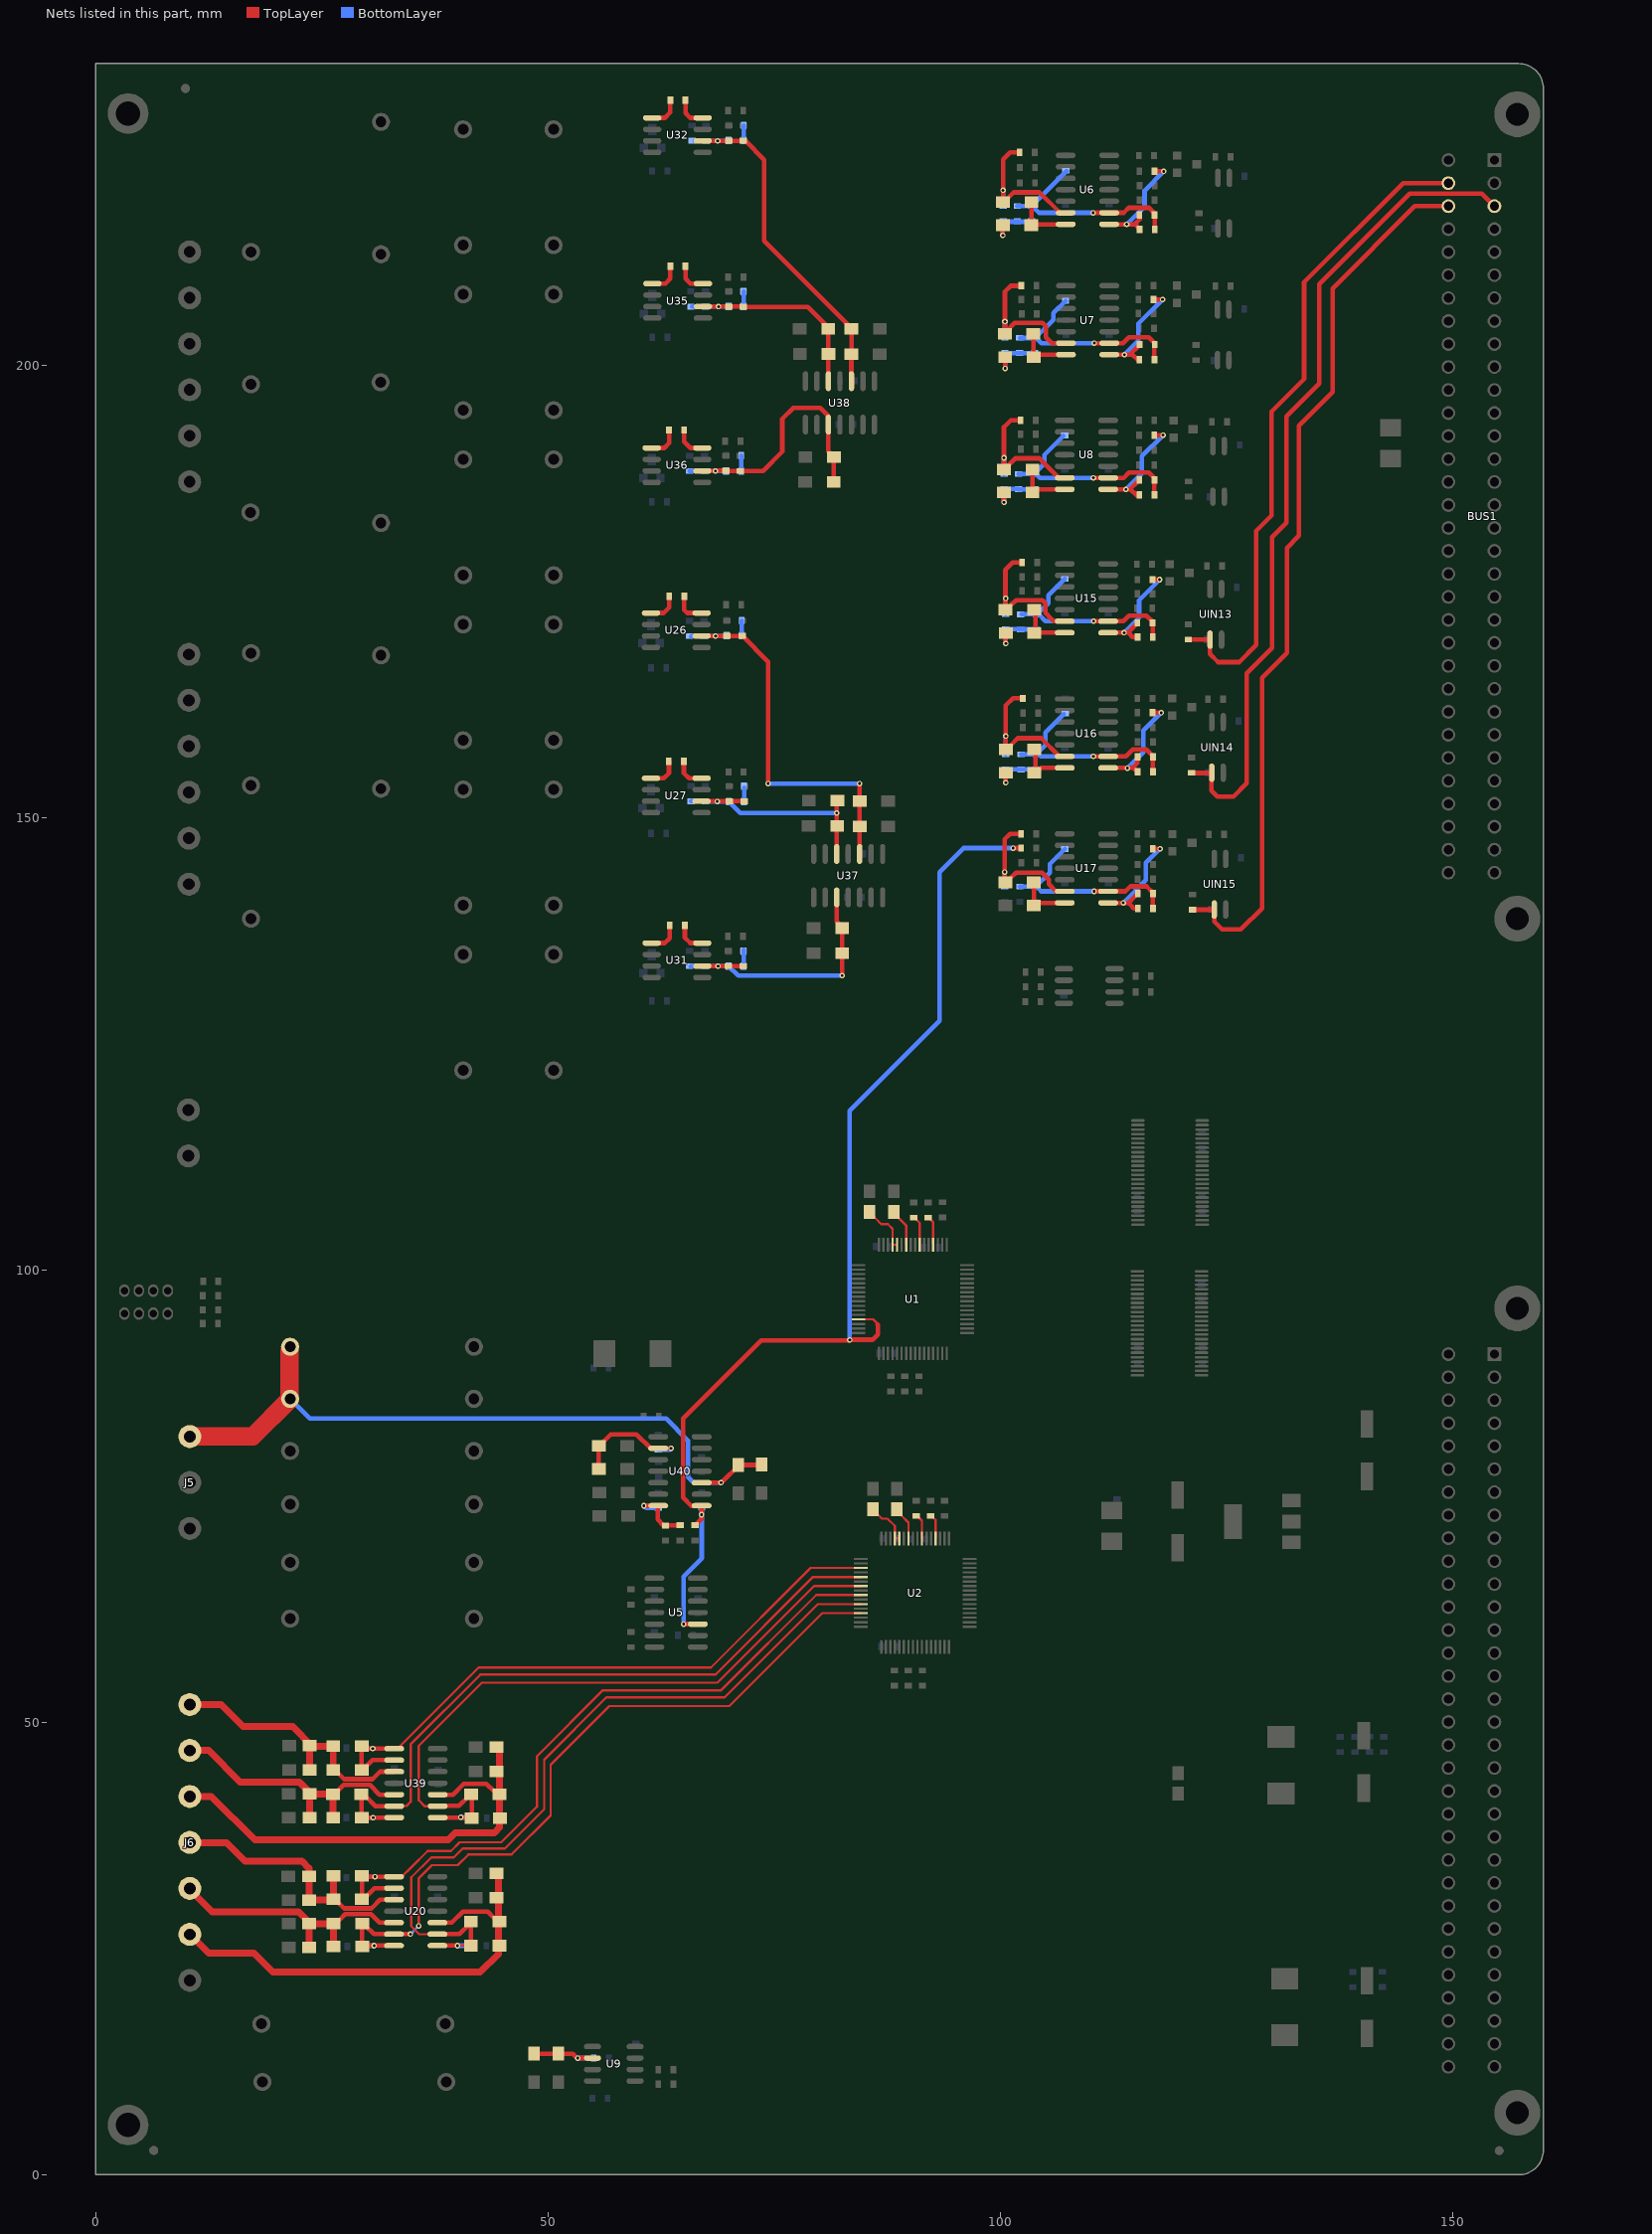
[diagram p0: the nets of this part, all layers, seen from the top]
# Altium PCB MISC80584.PCBDoc (part 5 of 7)
Units mm, origin at the board's own origin, x right, y up, seen from the top; angles counter-clockwise.
Board outline 160.02 x 233.3 mm, 4 copper layers (TopLayer, GND, POWER, BottomLayer); 386 components, 266 nets, 1374 pads, 640 vias.

## Via types
v1: diameter 0.61, hole 0.305, TopLayer to BottomLayer, 342 vias
v2: diameter 0.762, hole 0.381, TopLayer to BottomLayer, 197 vias
v3: diameter 0.508, hole 0.254, TopLayer to BottomLayer, 101 vias

## Nets (pads, with @x,y where several pads share a name; then routed paths per layer and width w, separated by ;. In a path a pad name is that pad's centre, name@x,y a point inside that pad or via, vN(x,y) a via of type N, cw(c..) or ccw(c..) an arc to the next point about the centre after c; other vN are vias at no path point) (continued)
ICC: C14.2 R85.1 R351.2 U1.61 U5.10 U40.8 | length 123.3
  TopLayer w0.254: U1.61@84.339,94.555 85.963,94.555 86.512,94.005
  TopLayer w0.508: v1(64.999,60.884) U5.10@66.56,60.884 ; C14.2@66.243,71.806 67.005,72.568 ; v1@67.005,72.974 67.005,73.939 66.98,73.965 65.837,73.965 64.948,74.854 64.948,83.617 73.558,92.227 83.261,92.227 83.337,92.304 85.877,92.304 86.462,92.888 86.462,93.548 86.462,93.955 86.436,93.98 ; v1(101.422,146.634) R351.2@102.286,146.634
  BottomLayer w0.254: R85.1@66.954,73.685 R85.1@66.98,73.66
  BottomLayer w0.508: v1(64.999,60.884) 64.999,66.142 67.005,68.148 R85.1@67.005,73.787 ; v1(83.363,92.278) 83.363,117.627 93.269,127.533 93.269,143.967 95.936,146.634 v1(101.422,146.634)
  other v1: 66.98,72.974
ICCIN: D95.K D97.A J5.1 R8.2 R9.2 U40.10 | length 78.5
  TopLayer w0.508: U40.10@66.992,76.505 v1(69.139,76.505) 69.164,76.505 71.12,78.461 D97.A@73.457,78.461
  TopLayer w2.032: J5.1@10.414,81.61 17.348,81.61 21.438,85.7 R9.2@21.438,91.034
  BottomLayer w0.508: R8.2@21.971,85.319 23.698,83.591 63.068,83.591 65.507,81.153 65.507,77.114 66.116,76.505 v1(69.139,76.505)
IILA: D28.K D33.A J6.1 R23.1 R24.1 U39.3 | length 29.4
  TopLayer w0.508: D33.A@26.67,44.577 27.495,43.752 30.594,43.752 31.42,44.577 U39.3@33.008,44.577
  TopLayer w0.762: J6.1@10.414,51.994 13.894,51.994 16.307,49.581 21.768,49.581 23.952,47.396 D28.K@26.264,47.396 D33.A@26.264,45.187 ; R24.1@23.622,47.117 23.673,47.066 R23.1@23.673,44.755
IILB: D26.K D31.A J6.2 R27.1 R29.1 U39.5 | length 29.5
  TopLayer w0.508: D31.A@26.746,42.443 27.407,43.104 30.328,43.104 31.394,42.037 U39.5@33.008,42.037
  TopLayer w0.762: J6.2@10.414,46.914 12.497,46.914 15.977,43.434 22.53,43.434 23.851,42.113 D31.A@26.162,42.113 ; R29.1@23.647,39.649 R27.1@23.647,42.113 ; D26.K@26.238,39.726 D31.A@26.238,42.062
IILC: D27.K D32.A J6.3 R32.1 R35.1 U39.10 | length 52.6
  TopLayer w0.508: U39.10@37.808,42.037 39.497,42.037 40.691,43.231 43.205,43.231 D32.A@44.044,42.393
  TopLayer w0.762: J6.3@10.414,41.834 12.802,41.834 17.602,37.033 38.989,37.033 39.776,37.821 44.069,37.821 44.653,38.405 R32.1@44.653,47.168
IISA: D62.K D65.A J6.4 R25.1 R26.1 U20.3 | length 29
  TopLayer w0.508: D65.A@26.721,30.226 27.483,29.464 30.485,29.464 30.582,29.56 30.582,29.566 31.445,30.429 U20.3@32.982,30.429
  TopLayer w0.762: J6.4@11.379,36.728 14.503,36.728 16.535,34.696 22.809,34.696 23.571,33.934 ; R26.1@23.597,32.868 23.597,33.934 ; R26.1@23.622,32.918 R25.1@23.622,30.378 26.162,30.378 26.314,30.531 D62.K@26.314,32.868
IISB: D63.K D80.A J6.5 R30.1 R31.1 U20.5 | length 28.8
  TopLayer w0.508: D63.K@26.949,28.194 27.572,28.816 30.442,28.816 31.369,27.889 U20.5@32.982,27.889
  TopLayer w0.762: J6.5@10.414,31.674 10.414,31.547 12.878,29.083 22.454,29.083 R31.1@23.749,27.788 ; R30.1@23.622,25.324 23.622,27.661 R31.1@23.749,27.788 ; R31.1@23.774,27.813 R31.1@23.749,27.788 ; D80.A@26.314,25.806 26.314,27.737 26.289,27.762 23.774,27.762 R31.1@23.749,27.788
IISC: D64.K D81.A J6.6 R36.1 R38.1 U20.10 | length 52.4
  TopLayer w0.508: U20.10@37.782,27.889 39.37,27.889 40.589,29.108 43.332,29.108 D81.A@44.018,28.423
  TopLayer w0.762: J6.6@10.414,26.594 12.497,24.511 17.526,24.511 19.609,22.428 42.52,22.428 44.526,24.435 R38.1@44.526,33.122
ILA: C12.2 D28.A D33.K U2.51 U39.1 U39.2 | length 70.3
  TopLayer w0.254: U39.1@33.376,47.117 42.342,56.083 68.021,56.083 79.032,67.094 U2.51@84.593,67.094
  TopLayer w0.508: D33.K@29.413,44.679 D33.K@29.413,44.78 29.413,47.117 30.607,47.117 v1(30.632,47.117) U39.1@33.008,47.117 U39.1@33.376,47.117 ; D33.K@29.947,45.187 30.607,45.847 U39.2@33.008,45.847
  BottomLayer w0.508: C12.2@29.54,47.117 v1(30.632,47.117)
ILB: C20.2 D26.A D31.K U2.53 U39.6 U39.7 | length 75.7
  TopLayer w0.254: U39.6@33.376,40.792 34.366,40.792 34.823,41.25 34.823,47.6 42.52,55.296 68.504,55.296 79.302,66.094 U2.53@84.593,66.094
  TopLayer w0.508: D26.A@29.312,39.929 29.388,40.005 D31.K@29.388,42.062 ; D31.K@29.82,41.885 30.937,40.767 U39.6@33.008,40.767 ; D26.A@29.87,39.522 29.896,39.497 U39.7@33.008,39.497
  BottomLayer w0.508: C20.2@29.413,39.497 v1(30.683,39.497)
ILC: C23.2 D27.A D32.K U2.55 U39.8 U39.9 | length 74.6
  TopLayer w0.254: U39.9@37.186,40.742 36.398,40.742 35.712,41.427 35.712,47.422 42.697,54.407 68.732,54.407 79.419,65.094 U2.55@84.593,65.094
  TopLayer w0.508: U39.8@37.808,39.497 v1@40.361,39.497 ; U39.9@38.43,40.792 40.183,40.792 41.123,41.732 41.529,41.732 41.58,41.681 41.58,39.522 41.554,39.497 v1@40.361,39.497 ; v1(40.361,39.548) v1@40.361,39.497
  BottomLayer w0.508: v1(40.361,39.548) 40.386,39.522 C23.2@41.478,39.522
IPR1: BUS1.C2 R600.2 UIN13.3 | length 72.8
  TopLayer w0.508: R600.2@120.777,169.672 123.139,169.672 UIN13.3@123.165,169.647 ; UIN13.3@123.165,169.443 123.165,168.097 124.079,167.183 126.39,167.183 128.27,169.062 128.27,181.686 129.972,183.388 129.972,194.869 133.579,198.476 133.579,209.169 144.526,220.116 BUS1.C2@149.53,220.116
IPR2: BUS1.A3 R601.2 UIN14.3 | length 91.6
  TopLayer w0.508: R601.2@121.209,154.94 123.241,154.94 123.342,155.042 123.342,152.984 124.003,152.324 125.781,152.324 127.254,153.797 127.254,165.938 130.048,168.732 130.048,181 131.623,182.575 131.623,194.361 135.255,197.993 135.255,208.966 145.237,218.948 153.238,218.948 BUS1.A3@154.61,217.576
IPR3: BUS1.C3 R602.2 UIN15.3 | length 98.6
  TopLayer w0.508: R602.2@121.437,139.827 123.622,139.827 123.673,139.878 123.647,139.878 UIN15.3@123.647,139.852 123.647,138.506 124.511,137.643 126.594,137.643 128.93,139.979 128.93,165.456 131.674,168.199 131.674,179.807 133.02,181.153 133.02,193.319 136.728,197.028 136.728,208.483 145.821,217.576 BUS1.C3@149.53,217.576
ISA: C13.2 D62.A D65.K U2.57 U20.1 U20.2 | length 78.8
  TopLayer w0.254: U20.1@32.982,32.969 33.858,32.969 34.874,33.985 ; 35.001,34.112 34.874,33.985 ; U2.57@84.593,64.094 79.664,64.094 69.139,53.569 56.083,53.569 48.793,46.279 48.793,40.716 44.844,36.767 40.246,36.767 39.294,35.814 36.703,35.814 34.874,33.985
  TopLayer w0.508: D65.K@29.439,30.505 D62.A@29.439,32.893 ; D62.A@29.489,32.969 v1(30.886,32.969) U20.1@32.982,32.969 ; D65.K@29.947,30.81 30.836,31.699 U20.2@32.982,31.699
  BottomLayer w0.508: C13.2@29.388,32.868 29.464,32.944 v1@30.886,32.944
ISB: C21.2 D63.A D80.K U2.61 U20.6 U20.7 | length 87.1
  TopLayer w0.254: D80.K@29.693,25.349 32.969,25.349 U20.7@32.982,25.349 ; U20.6@32.969,26.492 U20.6@33.02,26.543 ; v1(35.712,27.534) 35.712,32.791 35.916,32.995 ; 35.738,32.817 35.916,32.995 ; U2.61@84.593,62.094 80.331,62.094 70.053,51.816 56.769,51.816 50.292,45.339 50.292,39.751 45.974,35.433 41.224,35.433 40.03,34.239 37.16,34.239 35.916,32.995
  TopLayer w0.508: U20.7@33.147,25.349 33.122,25.375 29.642,25.375 29.464,25.552 29.464,27.254 29.794,27.584 30.759,26.619 U20.6@32.982,26.619 v1@34.773,26.619
  BottomLayer w0.254: v1(34.798,26.619) v1(35.712,27.534)
  BottomLayer w0.508: C21.2@29.515,25.273 29.591,25.349 v1(30.785,25.349)
ISC: C27.2 D64.A D81.K U2.59 U20.8 U20.9 | length 87
  TopLayer w0.254: U20.9@37.541,26.619 35.763,26.619 34.9,27.483 34.9,32.893 37.109,35.103 39.599,35.103 40.589,36.093 45.237,36.093 49.581,40.437 49.581,45.898 56.464,52.781 69.52,52.781 79.832,63.094 U2.59@84.593,63.094 ; U20.8@37.782,25.349 37.795,25.362 U20.8@37.795,25.375 ; U20.8@38.456,25.375 v1@40.005,25.375 ; v1(40.005,25.349) v1@40.005,25.375 ; D64.A@41.478,25.375 41.199,25.375 v1@40.005,25.375
  TopLayer w0.508: U20.9@37.782,26.619 40.234,26.619 D81.K@41.326,27.711 ; U20.8@38.049,25.375 v1@40.005,25.375 ; D64.A@41.199,25.375 41.478,25.654 D81.K@41.478,27.991
  BottomLayer w0.508: v1(40.005,25.349) 41.377,25.349 C27.2@41.402,25.375
IU1: C104.1 C113.1 C139.2 D10.K D14.A R119.1 R120.1 U32.6 U38.3 | length 39.9
  TopLayer w0.508: U32.6@67.107,224.79 v1(68.758,224.79) C139.2@71.679,224.79 ; C139.2@71.577,224.815 C139.2@71.857,224.815 ; C139.2@71.857,224.765 73.914,222.707 73.914,213.741 83.566,204.089 83.566,201.32 D10.K@83.541,201.295 ; U38.3@83.541,198.234 D10.K@83.541,201.244
  BottomLayer w0.508: R120.1@66.192,224.79 R119.1@67.488,224.79 v1(68.758,224.79) 69.901,224.79 C113.1@69.926,224.815
IU2: C126.2 C142.1 C143.1 D24.K D29.A R110.1 R111.1 U35.6 U38.5 | length 24.7
  TopLayer w0.508: U35.6@67.132,206.477 C142.1@69.977,206.477 71.577,206.477 71.603,206.451 78.74,206.451 81.001,204.191 D29.A@81.001,201.244 U38.5@81.001,198.234
  BottomLayer w0.508: R111.1@65.913,206.477 R110.1@67.412,206.477 v1@68.885,206.477 ; v1(68.859,206.477) v1@68.885,206.477 ; C143.1@69.774,206.477 v1@68.885,206.477
IU3: C130.1 C132.1 C136.2 D25.K D30.A R105.1 R106.1 U36.6 U38.10 | length 29.3
  TopLayer w0.508: U36.6@67.589,188.316 v1(68.504,188.316) ; v1@68.631,188.316 68.656,188.341 C130.1@69.672,188.341 ; C130.1@69.901,188.316 C136.2@71.272,188.316 73.762,188.316 75.895,190.449 75.895,194.056 77.114,195.275 80.112,195.275 80.975,194.412 U38.10@80.975,194.005 ; U38.10@81.001,193.434 81.001,190.5 D25.K@81.585,189.916 ; D30.A@81.509,187.274 81.585,187.35 D25.K@81.585,189.916 ; D25.K@81.585,190.094 D25.K@81.585,189.916 ; D25.K@81.661,189.84 D25.K@81.585,189.916
  BottomLayer w0.508: R105.1@65.659,188.316 67.158,188.316 R106.1@67.208,188.265 ; R106.1@67.488,188.341 67.513,188.316 v1(68.504,188.316) C132.1@69.698,188.316
IUA: C82.1 C83.1 C85.2 D8.K D12.A R138.1 R139.1 U26.6 U37.3 | length 43.3
  TopLayer w0.508: U26.6@66.98,170.078 v1(68.529,170.078) C85.2@71.399,170.078 ; C85.2@71.476,170.104 74.346,167.234 v1(74.346,153.772) ; v1(84.43,153.772) 84.43,152.298 D12.A@84.531,152.197 ; U37.3@84.455,145.986 D8.K@84.455,149.047 84.455,151.663 D12.A@84.506,151.714
  BottomLayer w0.508: R138.1@65.837,170.028 65.862,170.053 68.504,170.053 v1(68.529,170.078) C83.1@69.748,170.078 ; v1(74.346,153.772) v1(84.43,153.772)
IUB: C88.1 C89.1 C93.2 D11.K D15.A R131.1 R133.1 U27.6 U37.5 | length 27.3
  TopLayer w0.508: U27.6@66.98,151.816 v1@68.732,151.816 ; v1(68.707,151.79) v1@68.732,151.816 ; C93.2@71.73,151.765 71.679,151.816 71.018,151.816 v1@68.732,151.816 ; D11.K@81.89,151.943 81.915,151.917 81.915,151.867 U37.5@81.915,145.986
  BottomLayer w0.508: R131.1@65.837,151.816 67.31,151.816 67.361,151.765 C89.1@69.926,151.765 ; C89.1@70.002,151.79 71.272,150.52 v1(81.915,150.52)
IUC: C96.1 C97.1 C101.2 D9.K D13.A R125.1 R126.1 U31.6 U37.10 | length 29.4
  TopLayer w0.508: U31.6@67.564,133.604 v1(68.809,133.604) ; v1@68.91,133.604 69.901,133.604 C96.1@69.952,133.553 ; C96.1@70.079,133.604 71.145,133.604 C101.2@71.577,133.604 ; U37.10@81.915,141.186 81.915,138.532 82.525,137.922 D9.K@82.525,137.795 D13.A@82.525,135.382 ; D13.A@82.474,134.976 82.525,134.925 v1(82.525,132.537)
  BottomLayer w0.508: R126.1@65.761,133.553 65.811,133.604 R125.1@67.335,133.604 v1(68.809,133.604) C97.1@69.799,133.604 ; C97.1@69.952,133.604 71.018,132.537 v1(82.525,132.537)
NetC4_1: C4.1 R150.2 R450.1 U6.8 | length 13.6
  TopLayer w0.508: U6.8@112.026,215.57 v1(113.97,215.57) 114.884,215.57 114.91,215.544 ; 114.859,215.595 114.91,215.646 ; R450.1@115.392,216.687 115.392,216.129 114.91,215.646 ; C4.1@115.443,215.011 114.91,215.544 ; R150.2@117.043,221.412 v1(118.059,221.412) ; 114.91,215.544 114.91,215.646
  BottomLayer w0.508: v1(113.97,215.57) 115.951,217.551 115.951,219.304 v1(118.059,221.412)
NetC4_2: C4.2 R76.1 R100.1 R132.1 R450.2 U6.9 | length 22.7
  TopLayer w0.508: v1(110.261,216.84) U6.9@112.026,216.84 113.64,216.84 114.198,217.399 116.434,217.399 117.069,216.764 C4.2@117.069,215.316
  BottomLayer w0.508: R132.1@101.879,217.576 R100.1@103.429,217.576 ; R100.1@103.454,217.576 107.315,221.437 R76.1@107.366,221.437 ; R100.1@103.632,217.475 104.267,216.84 v1(110.261,216.84)
NetC5_1: C5.1 R151.2 R451.1 U7.8 | length 13.6
  TopLayer w0.508: U7.8@112.052,201.168 v1(113.716,201.168) 114.605,201.168 115.138,200.635 C5.1@115.443,200.635 ; 114.351,201.193 R451.1@115.24,202.082 ; R151.2@117.043,207.239 117.907,207.239 v1(117.932,207.264)
  BottomLayer w0.508: v1(113.716,201.168) 115.265,202.717 115.265,204.597 v1(117.932,207.264)
NetC5_2: C5.2 R86.1 R108.1 R146.1 R451.2 U7.9 | length 22.7
  TopLayer w0.508: v1(110.388,202.438) U7.9@112.052,202.438 113.563,202.438 114.211,203.086 116.395,203.086 117.018,202.463 C5.2@117.018,200.66
  BottomLayer w0.508: R146.1@102.21,202.997 103.861,202.997 105.867,205.003 105.867,205.765 R86.1@107.213,207.112 ; R108.1@104.013,202.971 104.546,202.438 v1(110.388,202.438)
NetC6_1: C6.1 R152.2 R452.1 U8.8 | length 13.5
  TopLayer w0.508: U8.8@111.925,186.284 114.3,186.284 R452.1@115.189,187.173 ; 114.402,186.284 115.037,185.649 C6.1@115.367,185.649 ; R152.2@117.018,192.278 v1(117.983,192.278)
  BottomLayer w0.508: v1(113.894,186.284) 115.646,188.036 115.646,189.941 v1(117.983,192.278)
NetC6_2: C6.2 R87.1 R117.1 R147.1 R452.2 U8.9 | length 22.6
  TopLayer w0.508: v1(110.287,187.554) U8.9@111.925,187.554 113.64,187.554 114.211,188.125 116.421,188.125 117.018,187.528 C6.2@117.018,185.877
  BottomLayer w0.508: R147.1@102.032,187.985 103.734,187.985 104.877,189.128 104.877,190.094 R87.1@106.959,192.176 ; R117.1@103.988,187.935 104.369,187.554 v1(110.287,187.554)
NetC11_2: C11.2 R5.2 R93.1 U40.7 | length 7.4
  TopLayer w0.508: v1(60.604,73.965) U40.7@62.192,73.965 ; U40.7@62.128,73.812 62.128,72.441 62.763,71.806 C11.2@64.618,71.806
  BottomLayer w0.508: v1@60.63,73.965 60.858,73.736 R93.1@62.179,73.736
NetC15_1: C15.1 R375.2 R459.1 U15.8 | length 12.8
  TopLayer w0.508: U15.8@111.925,170.434 114.097,170.434 C15.1@114.986,171.323 ; 114.249,170.332 114.605,169.977 R459.1@115.164,169.977 ; R375.2@116.815,176.301 v1(117.602,176.301)
  BottomLayer w0.508: v1(113.69,170.434) 115.341,172.085 115.341,174.041 v1(117.602,176.301)
NetC15_2: C15.2 R360.1 R364.1 R372.1 R459.2 U15.9 | length 21.6
  TopLayer w0.508: v1(110.312,171.704) U15.9@111.354,171.704 ; U15.9@111.925,171.704 113.589,171.704 114.224,172.339 116.154,172.339 116.84,171.653 R459.2@116.84,170.002
  BottomLayer w0.508: R364.1@102.362,172.466 R372.1@104.013,172.466 R372.1@104.064,172.466 ; R360.1@107.112,176.378 105.308,174.574 105.308,173.711 R372.1@104.064,172.466 ; v1(110.312,171.704) 105.004,171.704 104.242,172.466 R372.1@104.064,172.466
NetC16_1: C16.1 R376.2 R460.1 U16.8 | length 13
  TopLayer w0.508: U16.8@111.925,155.499 v1@114.021,155.499 ; v1(114.046,155.473) v1@114.021,155.499 ; 114.681,155.575 115.138,156.032 115.138,156.667 R460.1@115.189,156.718 ; C16.1@114.986,155.245 114.732,155.499 v1@114.021,155.499 ; R376.2@116.967,161.595 v1(117.78,161.595)
  BottomLayer w0.508: v1(114.046,155.473) 115.799,157.226 115.799,159.614 v1(117.78,161.595)
NetC16_2: C16.2 R361.1 R365.1 R373.1 R460.2 U16.9 | length 22.5
  TopLayer w0.508: v1(110.287,156.769) U16.9@111.925,156.769 113.894,156.769 114.656,157.531 116.154,157.531 116.764,156.921 116.764,156.87 116.84,156.794 C16.2@116.84,155.143
  BottomLayer w0.508: R365.1@102.311,156.997 103.988,156.997 R373.1@104.013,157.023 105.004,158.013 105.004,159.41 R361.1@107.036,161.442 ; R373.1@104.165,157.074 104.47,156.769 v1(110.287,156.769)
NetC17_1: C17.1 R377.2 R461.1 U17.8 | length 13
  TopLayer w0.508: U17.8@111.925,140.589 114.173,140.589 R461.1@115.011,141.427 ; 114.275,140.487 114.783,139.979 C17.1@115.214,139.979 ; R377.2@116.84,146.558 v1(117.653,146.558)
  BottomLayer w0.508: v1(113.589,140.589) 116.103,143.104 116.103,144.323 116.103,145.009 v1(117.653,146.558)
NetC17_2: C17.2 R362.1 R366.1 R374.1 R461.2 U17.9 | length 22.3
  TopLayer w0.508: v1(110.363,141.859) U17.9@111.925,141.859 113.843,141.859 114.389,142.405 116.167,142.405 116.84,141.732 C17.2@116.84,140.132
  BottomLayer w0.508: R374.1@102.159,142.392 R366.1@103.835,142.392 103.911,142.392 105.461,143.942 105.461,144.882 R362.1@107.112,146.533 ; R366.1@104.038,142.342 104.521,141.859 v1(110.363,141.859)
NetC19_2: C19.2 U1.39 | length 3
  TopLayer w0.254: C19.2@90.678,105.639 91.089,105.228 U1.39@91.089,102.805
NetC22_2: C22.2 U1.36 | length 3.1
  TopLayer w0.254: C22.2@92.151,105.715 92.589,105.277 U1.36@92.589,102.805
NetC25_2: C25.2 U2.39 | length 2.6
  TopLayer w0.254: C25.2@90.907,72.746 91.343,72.31 U2.39@91.343,70.344
NetC26_2: C26.2 U2.36 | length 2.4
  TopLayer w0.254: C26.2@92.583,72.644 92.837,72.39 92.837,71.869 92.835,71.866 92.835,70.352 U2.36@92.843,70.344
NetC83_2: C83.2 R137.1 | length 1.7
  BottomLayer w0.508: R137.1@71.425,171.78 71.425,170.688 71.425,170.129 C83.2@71.45,170.104
NetC84_1: C84.1 U26.8 | length 3.4
  TopLayer w0.508: C84.1@65.049,174.32 65.049,172.949 65.38,172.618 U26.8@66.98,172.618
NetC84_2: C84.2 U26.1 | length 3.4
  TopLayer w0.508: U26.1@61.392,172.618 62.789,172.618 63.398,173.228 C84.2@63.398,174.371
NetC89_2: C89.2 R130.1 | length 1.5
  BottomLayer w0.508: C89.2@71.679,151.79 71.679,152.298 R130.1@71.679,153.289
NetC92_1: C92.1 U27.8 | length 3.5
  TopLayer w0.508: C92.1@65.024,156.185 65.024,154.915 65.583,154.356 U27.8@66.98,154.356
NetC92_2: C92.2 U27.1 | length 3.5
  TopLayer w0.508: U27.1@61.392,154.356 62.814,154.356 63.373,154.915 C92.2@63.373,156.21
NetC97_2: C97.2 R124.1 | length 1.8
  BottomLayer w0.508: C97.2@71.628,133.604 71.628,134.264 R124.1@71.628,135.255 R124.1@71.628,135.382
NetC100_1: C100.1 U31.8 | length 3.6
  TopLayer w0.508: C100.1@65.126,138.125 C100.1@65.126,138.1 65.126,136.754 65.735,136.144 U31.8@67.056,136.144
NetC100_2: C100.2 U31.1 | length 3.5
  TopLayer w0.508: U31.1@61.468,136.144 62.916,136.144 63.449,136.677 C100.2@63.449,137.998
NetC113_2: C113.2 R118.1 | length 1.7
  BottomLayer w0.508: C113.2@71.628,224.765 71.653,224.79 C113.2@71.653,224.815 71.653,225.577 R118.1@71.653,226.492
NetC118_1: C118.1 U32.8 | length 3.4
  TopLayer w0.508: C118.1@65.227,229.184 65.227,227.838 65.735,227.33 U32.8@67.107,227.33
NetC118_2: C118.2 U32.1 | length 3.6
  TopLayer w0.508: U32.1@61.519,227.33 62.916,227.33 63.525,227.94 C118.2@63.525,229.286 C118.2@63.525,229.311
NetC121_2: C121.2 U1.44 U1.45 | length 4.8
  TopLayer w0.254: C121.2@86.081,105.842 86.843,105.08 87.579,105.08 88.101,104.558 88.101,102.805 U1.44@88.589,102.805
NetC122_2: C122.2 U1.42 | length 3.6
  TopLayer w0.254: C122.2@88.544,105.994 89.589,104.95 U1.42@89.589,102.805
NetC123_2: C123.2 U2.44 U2.45 | length 4.4
  TopLayer w0.254: C123.2@86.411,73.05 86.919,72.542 87.528,72.542 88.343,71.728 U2.45@88.343,70.357 ; U2.45@88.341,70.358 U2.45@88.343,70.357 ; U2.45@88.343,70.344 U2.45@88.343,70.357 ; U2.44@88.843,70.344 88.355,70.344 U2.45@88.343,70.357
NetC124_2: C124.2 U2.42 | length 3
  TopLayer w0.254: C124.2@89.002,72.949 89.843,72.108 U2.42@89.843,70.344
NetC125_1: C125.1 U35.8 | length 3.5
  TopLayer w0.508: C125.1@65.202,210.896 65.202,209.55 65.735,209.017 U35.8@67.132,209.017
NetC125_2: C125.2 U35.1 | length 3.5
  TopLayer w0.508: U35.1@61.544,209.017 62.992,209.017 63.525,209.55 C125.2@63.525,210.82
NetC132_2: C132.2 R414.1 | length 1.7
  BottomLayer w0.508: C132.2@71.374,188.29 C132.2@71.374,188.316 R414.1@71.374,189.992
NetC135_1: C135.1 U36.8 | length 3.6
  TopLayer w0.508: C135.1@65.049,192.837 65.049,191.567 65.761,190.856 U36.8@67.056,190.856
NetC135_2: C135.2 U36.1 | length 3.4
  TopLayer w0.508: U36.1@61.468,190.856 62.84,190.856 63.398,191.414 C135.2@63.398,192.684
NetC143_2: C143.2 R113.1 | length 1.7
  BottomLayer w0.508: C143.2@71.628,206.477 R113.1@71.628,208.153
NetD1_A: D1.A D2.K R11.2 U9.2 | length 8.1
  TopLayer w0.508: D2.K@48.768,13.386 52.73,13.386 53.188,12.929 U9.2@54.927,12.929
  BottomLayer w0.508: v1(53.289,12.929) R11.2@54.991,12.929
NetD16_A: D16.A D20.K U6.7 | length 5.5
  TopLayer w0.508: D16.A@103.454,218.034 103.454,215.697 103.581,215.57 U6.7@106.578,215.57
NetD16_K: D16.K R57.1 R67.2 U6.6 | length 15.8
  TopLayer w0.508: D16.K@100.305,218.415 100.305,222.733 101.092,223.52 R57.1@102.133,223.52 ; D16.K@100.813,218.44 101.473,219.1 104.343,219.1 106.604,216.84 U6.6@107.226,216.84
  BottomLayer w0.508: R67.2@100.305,217.576 v1(100.305,219.329)
NetD17_A: D17.A D21.K U7.7 | length 5.7
  TopLayer w0.508: D17.A@103.657,203.479 103.657,201.066 103.708,201.016 103.861,201.168 U7.7@106.883,201.168
NetD17_K: D17.K R58.1 R70.2 U7.6 | length 17.1
  TopLayer w0.508: D17.K@100.508,203.479 100.508,208.128 101.143,208.763 R58.1@102.26,208.763 ; D17.K@100.686,203.759 101.6,204.673 104.673,204.673 105.029,204.318 105.029,203.098 105.689,202.438 U7.6@107.252,202.438
  BottomLayer w0.508: R70.2@100.508,203.022 v1(100.508,204.826)
NetD18_A: D18.A D22.K U8.7 | length 5.3
  TopLayer w0.508: D18.A@103.556,188.519 103.556,186.309 D22.K@103.607,186.258 ; D22.K@104.115,186.284 U8.7@107.125,186.284
NetD18_K: D18.K R59.1 R71.2 U8.6 | length 16.2
  TopLayer w0.508: D18.K@100.406,188.519 100.406,193.167 101.168,193.929 R59.1@102.108,193.929 ; D18.K@100.711,188.747 101.676,189.713 104.298,189.713 104.699,189.312 104.699,189.306 106.451,187.554 U8.6@107.125,187.554
  BottomLayer w0.508: R71.2@100.406,187.985 v1(100.406,189.763)
NetD20_A: D20.A R67.1 R100.2 R132.2 | length 5.8
  TopLayer w0.508: v1(100.279,214.351) D20.A@100.279,215.468
  BottomLayer w0.508: v1(100.279,214.351) R67.1@100.279,215.849 ; R67.1@100.279,215.875 100.305,215.849 103.403,215.849 R100.2@103.454,215.9
NetD21_A: D21.A R70.1 R108.2 R146.2 | length 6.1
  TopLayer w0.508: v1(100.533,199.644) D21.A@100.533,200.889
  BottomLayer w0.508: R70.1@100.508,201.346 R70.1@100.533,201.32 ; v1(100.533,199.644) R70.1@100.533,201.32 ; R70.1@100.533,201.346 R70.1@100.533,201.32 ; R108.2@103.632,201.32 R70.1@100.533,201.32
NetD22_A: D22.A R71.1 R117.2 R147.2 | length 5.9
  TopLayer w0.508: v1(100.406,184.836) D22.A@100.406,185.953
  BottomLayer w0.508: v1(100.406,184.836) R71.1@100.406,186.207 ; R71.1@100.406,186.309 101.981,186.309 102.006,186.284 R117.2@103.81,186.284
NetD60_A: D60.A D61.K R97.2 U40.2 | length 13.4
  TopLayer w0.508: D61.K@55.601,77.826 55.601,80.518 56.947,81.864 59.792,81.864 61.366,80.289 U40.2@62.052,80.289 ; U40.2@62.052,80.315 U40.2@62.192,80.315 v1(63.602,80.315)
  BottomLayer w0.508: R97.2@62.205,80.162 63.5,80.162 v1@63.627,80.289
NetD83_A: D83.A D89.K U15.7 | length 5.7
  TopLayer w0.508: D83.A@103.861,172.923 103.886,172.898 103.886,170.459 103.911,170.434 U15.7@107.125,170.434
NetD83_K: D83.K R353.1 R357.2 U15.6 | length 15.7
  TopLayer w0.508: D83.K@100.559,173.304 100.559,177.394 101.346,178.181 R353.1@102.413,178.181 ; D83.K@101.194,173.507 101.727,174.041 104.646,174.041 104.889,173.797 104.889,173.78 104.968,173.701 104.968,172.628 105.588,172.009 105.893,171.704 U15.6@107.125,171.704
  BottomLayer w0.508: R357.2@100.584,172.517 v1(100.584,174.219)
NetD84_A: D84.A D90.K U16.7 | length 5.5
  TopLayer w0.508: D84.A@103.81,157.378 103.886,157.302 103.886,155.194 D90.K@104.292,155.194 ; D90.K@104.292,155.296 104.496,155.499 U16.7@107.125,155.499
NetD84_K: D84.K R354.1 R358.2 U16.6 | length 16.1
  TopLayer w0.508: D84.K@100.609,157.556 v1(100.609,159.004) 100.609,162.408 101.397,163.195 R354.1@102.438,163.195 ; D84.K@101.168,158.013 101.93,158.775 104.521,158.775 106.528,156.769 U16.6@107.125,156.769
  BottomLayer w0.508: R358.2@100.609,157.023 v1(100.609,159.004)
NetD85_A: D85.A D91.K U17.7 | length 5.4
  TopLayer w0.508: D85.A@103.734,142.697 103.734,140.818 103.988,140.564 104.013,140.589 U17.7@107.125,140.589
NetD85_K: D85.K R355.1 R359.2 U17.6 | length 15.4
  TopLayer w0.508: D85.K@100.482,143.205 100.482,147.625 101.067,148.209 R355.1@102.286,148.209 ; D85.K@101.168,143.358 101.727,143.916 104.603,143.916 105.359,143.16 105.359,142.646 106.147,141.859 U17.6@107.125,141.859
  BottomLayer w0.508: R359.2@100.482,142.418 v1(100.482,143.993)
NetD89_A: D89.A R357.1 R364.2 R372.2 | length 6.2
  TopLayer w0.508: v1(100.609,169.24) D89.A@100.609,170.409
  BottomLayer w0.508: R357.1@100.584,170.84 102.083,170.84 102.108,170.815 R372.2@104.089,170.815 ; v1(100.609,169.24) R357.1@100.609,170.764
NetD90_A: D90.A R358.1 R365.2 R373.2 | length 5.8
  TopLayer w0.508: v1(100.609,153.873) D90.A@100.609,155.016
  BottomLayer w0.508: v1(100.609,153.873) R358.1@100.609,155.219 ; R358.1@100.609,155.346 R373.2@103.886,155.346